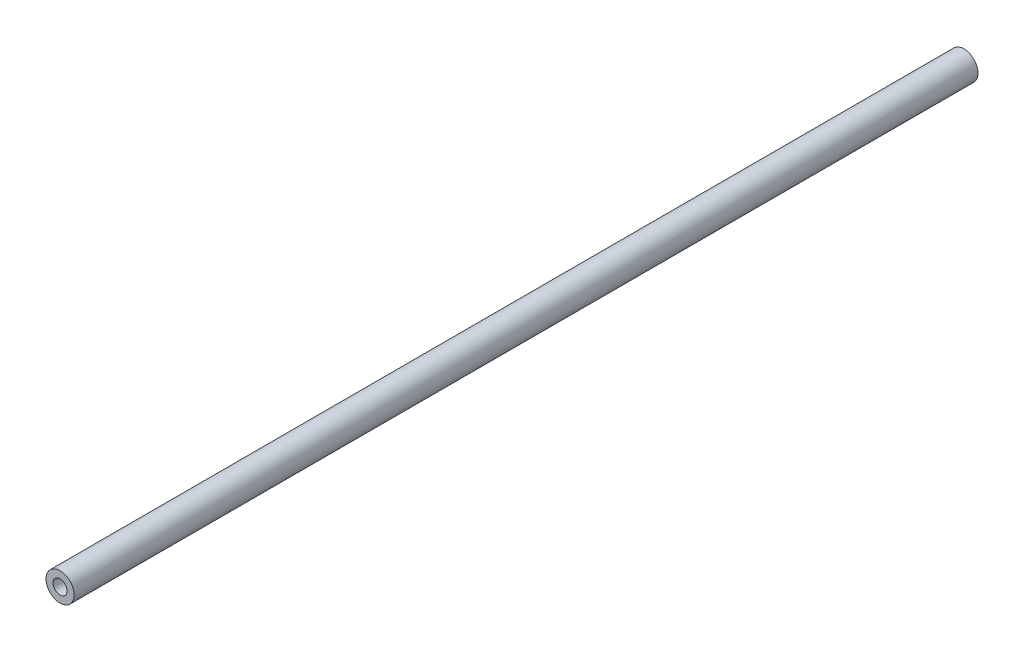
SolidWorks part; units mm, degrees
ref_plane "Front Plane" through (0, 0, 0) normal (0, 0, 1) x (1, 0, 0)
ref_plane "Top Plane" through (0, 0, 0) normal (0, 1, 0) x (1, 0, 0)
ref_plane "Right Plane" through (0, 0, 0) normal (1, 0, 0) x (0, 0, -1)
sketch "Sketch1" plane through (0, 0, 0) normal (0, 0, 1) x (1, 0, 0)
  circle A0 centre (0, 0) radius 5
  dimension "D1" = 10
extrude "Boss-Extrude1" add sketch "Sketch1" along normal blind 321
hole_wizard "M6 Tapped Hole1" positions "Sketch2" profile "Sketch3" tap size "M6" standard "GB"
sketch "Sketch2" plane through (0, 0, 321) normal (0, 0, 1) x (1, 0, 0)
  point P0 (0, 0)
sketch "Sketch3" plane through (0, 0, 321) normal (1, 0, 0) x (0, -1, 0)
  line L0 (0, 0) -> (0, 16.5022)
  line L1 (0, 16.5022) -> (2.5, 15)
  line L2 (2.5, 15) -> (2.5, 0)
  line L5 (2.5, 0) -> (0, 0)
  line L10 (0, 16.5022) -> (-2.5, 15) construction
  line L11 (0, -6.35) -> (0, 107.95) construction
  dimension "螺纹孔钻头直径" = 5
  dimension "螺纹孔钻头深度" = 15
  dimension "导头角度" = 118
cosmetic thread "Cosmetic Thread1" parameters "D1"=12, "D2"=6
hole_wizard "M6 Tapped Hole2" positions "Sketch4" profile "Sketch5" tap size "M6" standard "GB"
sketch "Sketch4" plane through (0, 0, 0) normal (0, 0, -1) x (-1, 0, 0)
  point P0 (0, 0)
sketch "Sketch5" plane through (0, 0, 0) normal (1, 0, 0) x (0, 1, 0)
  line L0 (0, 0) -> (0, 16.5022)
  line L1 (0, 16.5022) -> (2.5, 15)
  line L2 (2.5, 15) -> (2.5, 0)
  line L5 (2.5, 0) -> (0, 0)
  line L10 (0, 16.5022) -> (-2.5, 15) construction
  line L11 (0, -6.35) -> (0, 107.95) construction
  dimension "螺纹孔钻头直径" = 5
  dimension "螺纹孔钻头深度" = 15
  dimension "导头角度" = 118
cosmetic thread "Cosmetic Thread2" parameters "D1"=12, "D2"=6
